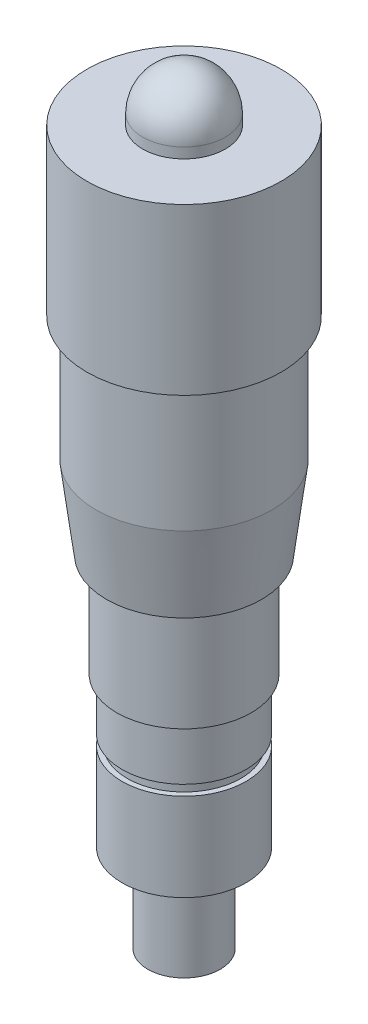
SolidWorks part; units mm, degrees
ref_plane "Front Plane" through (0, 0, 0) normal (0, 0, 1) x (1, 0, 0)
ref_plane "Top Plane" through (0, 0, 0) normal (0, 1, 0) x (1, 0, 0)
ref_plane "Right Plane" through (0, 0, 0) normal (1, 0, 0) x (0, 0, -1)
sketch "Sketch1" plane through (0, 0, 0) normal (0, 1, 0) x (1, 0, 0)
  circle A0 centre (0, 0) radius 1.75
  dimension "D1" = 3.5
extrude "Boss-Extrude1" add sketch "Sketch1" along normal blind 4.25
sketch "Sketch2" plane through (0, 4.25, 0) normal (0, 1, 0) x (1, 0, 0)
  circle A0 centre (0, 0) radius 3
  dimension "D1" = 6
extrude "Boss-Extrude2" add sketch "Sketch2" along normal blind 4.25
sketch "Sketch3" plane through (0, 8.5, 0) normal (0, 1, 0) x (1, 0, 0)
  circle A0 centre (0, 0) radius 2.75
  dimension "D1" = 5.5
extrude "Boss-Extrude3" add sketch "Sketch3" along normal blind 0.5
sketch "Sketch4" plane through (0, 9, 0) normal (0, 1, 0) x (1, 0, 0)
  circle A0 centre (0, 0) radius 3
  dimension "D1" = 6
extrude "Boss-Extrude4" add sketch "Sketch4" along normal blind 2.5
sketch "Sketch5" plane through (0, 11.5, 0) normal (0, 1, 0) x (1, 0, 0)
  circle A0 centre (0, 0) radius 3.25
  dimension "D1" = 6.5
extrude "Boss-Extrude5" add sketch "Sketch5" along normal blind 5
sketch "Sketch6" plane through (0, 16.5, 0) normal (0, 1, 0) x (1, 0, 0)
  circle A0 centre (0, 0) radius 4.25
  dimension "D1" = 8.5
extrude "Boss-Extrude6" add sketch "Sketch6" along normal blind 10
chamfer "Chamfer1" distance 0.5 distance2 4 1 edges at (0, 16.5, 4.25)
sketch "Sketch7" plane through (0, 26.5, 0) normal (0, 1, 0) x (1, 0, 0)
  circle A0 centre (0, 0) radius 4.7
  dimension "D1" = 9.4
extrude "Boss-Extrude7" add sketch "Sketch7" along normal blind 8
sketch "Sketch8" plane through (0, 34.5, 0) normal (0, 1, 0) x (1, 0, 0)
  circle A0 centre (0, 0) radius 2
  dimension "D1" = 4
extrude "Boss-Extrude8" add sketch "Sketch8" along normal blind 2.5
fillet "Fillet1" radius 2 1 edges at (0, 37, 2)
